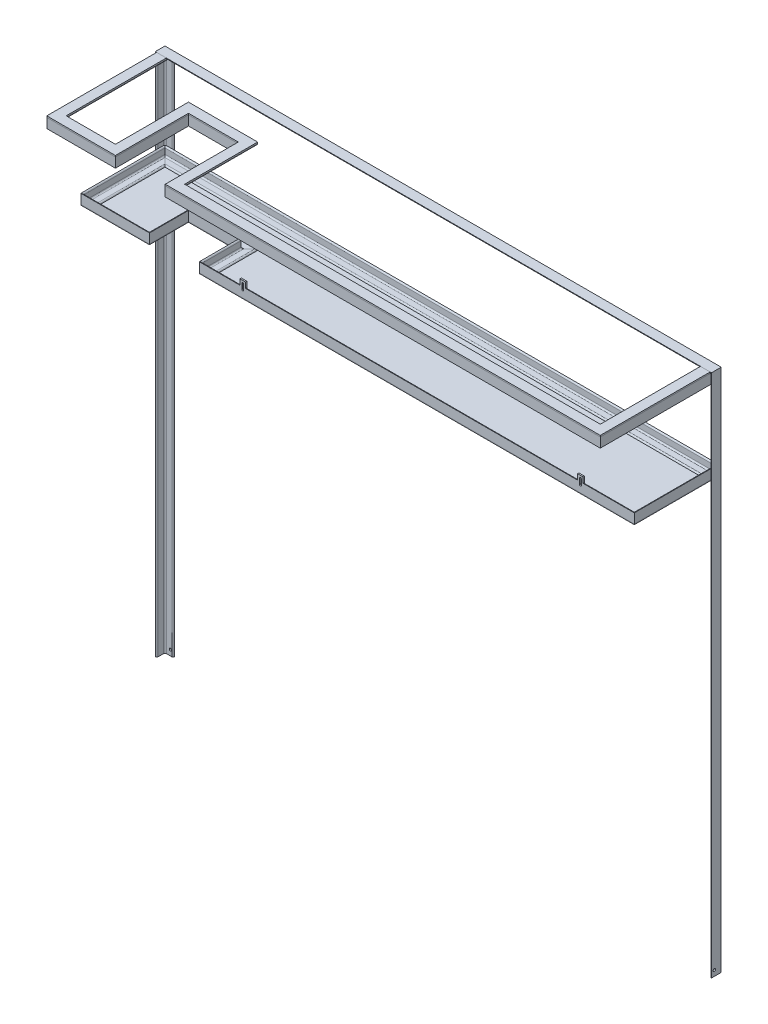
from build123d import *

# Parameters (mm, degrees)
MEMBER_1_DEPTH        = 1944.497474683
MEMBER_1_2_DEPTH      = 2060.497474683
MEMBER_1_2_DEPTH_BACK = 50.497474683
MEMBER_1_3_DEPTH      = 1944.497474683
MEMBER_2_DEPTH        = 477.497474683
MEMBER_2_2_DEPTH      = 348.994949366
MEMBER_2_3_DEPTH      = 364.994949366
MEMBER_2_4_DEPTH      = 280.994949366
MEMBER_2_5_DEPTH      = 364.994949366
MEMBER_2_6_DEPTH      = 1672.994949366
MEMBER_2_7_DEPTH      = 477.497474683
MEMBER_3_DEPTH        = 354.497474683
MEMBER_3_DEPTH_BACK   = 50.497474683
MEMBER_3_2_DEPTH      = 1672.994949366
MEMBER_3_3_DEPTH      = 241.994949366
MEMBER_3_4_DEPTH      = 280.994949366
MEMBER_3_5_DEPTH      = 241.994949366
MEMBER_3_6_DEPTH      = 348.994949366
MEMBER_3_7_DEPTH      = 404.994949366
MEMBER_3_8_DEPTH      = 2100.994949366
SKETCH_8_R            = 4.5
CUT_EXTRUDE_1_DEPTH   = 10
CUT_EXTRUDE_START     = -50
SKETCH_9_R            = 4.5
CUT_EXTRUDE_2_DEPTH   = 2440
EXTRUDE_1_DEPTH       = 5
EXTRUDE_2_DEPTH       = 2
SKETCH_14_W           = 20
SKETCH_14_H           = 30
EXTRUDE_3_DEPTH       = 5
CUT_EXTRUDE_3_DEPTH   = 5


with BuildPart() as part:
    # Sketch1 on segment 1 (carried to segment 1) → Member 1 (new body)
    with BuildSketch(Plane.ZX.offset(-1894)):
        with BuildLine():
            Line((0, 0), (0, 35))
            ThreePointArc((0, 35), (3.535533906, 33.535533906), (5, 30))
            Line((5, 30), (5, 10))
            ThreePointArc((5, 10), (6.464466094, 6.464466094), (10, 5))
            Line((10, 5), (30, 5))
            ThreePointArc((30, 5), (33.535533906, 3.535533906), (35, 0))
            Line((35, 0), (0, 0))
        make_face()
    extrude(amount=MEMBER_1_DEPTH)

    # Member 1 mitre 1
    split(bisect_by=Plane(origin=(0, 0, 0), x_dir=(0.707106781, -0.707106781, 0), z_dir=(-0.707106781, -0.707106781, 0)), keep=Keep.TOP)

    # 草图8 → 切除-拉伸1 (cut)
    with BuildSketch(Plane.XY.offset(5)):
        with Locations((25, -1874)):
            Circle(SKETCH_8_R)
        with Locations((2413, -1874)):
            Circle(SKETCH_8_R)
    extrude(amount=-CUT_EXTRUDE_1_DEPTH, mode=Mode.SUBTRACT)


with BuildPart() as body_2:
    # Sketch1 → Member 1 2 (new, two sides: drawn at the far end of the back side and taken through both)
    with BuildSketch(Plane(origin=(0, 0, 0), x_dir=(0, 0, 1), z_dir=(1, 0, 0)).offset(-MEMBER_1_2_DEPTH_BACK)):
        with BuildLine():
            Line((0, 0), (0, 35))
            ThreePointArc((0, 35), (3.535533906, 33.535533906), (5, 30))
            Line((5, 30), (5, 10))
            ThreePointArc((5, 10), (6.464466094, 6.464466094), (10, 5))
            Line((10, 5), (30, 5))
            ThreePointArc((30, 5), (33.535533906, 3.535533906), (35, 0))
            Line((35, 0), (0, 0))
        make_face()
    extrude(amount=MEMBER_1_2_DEPTH + MEMBER_1_2_DEPTH_BACK)

    # Member 1 2 mitre 1
    split(bisect_by=Plane(origin=(0, 0, 0), x_dir=(-0.707106781, 0.707106781, 0), z_dir=(0.707106781, 0.707106781, 0)), keep=Keep.TOP)

    # Member 1 2 mitre 2
    split(bisect_by=Plane(origin=(2010, 0, 0), x_dir=(-0.707106781, -0.707106781, 0), z_dir=(-0.707106781, 0.707106781, 0)), keep=Keep.TOP)


with BuildPart() as body_3:
    # Sketch1 on segment 3 (carried to segment 3) → Member 1 3 (new body)
    with BuildSketch(Plane(origin=(2010, 50.497474683, 0), x_dir=(0, 0, 1), z_dir=(0, -1, 0))):
        with BuildLine():
            Line((0, 0), (0, 35))
            ThreePointArc((0, 35), (3.535533906, 33.535533906), (5, 30))
            Line((5, 30), (5, 10))
            ThreePointArc((5, 10), (6.464466094, 6.464466094), (10, 5))
            Line((10, 5), (30, 5))
            ThreePointArc((30, 5), (33.535533906, 3.535533906), (35, 0))
            Line((35, 0), (0, 0))
        make_face()
    extrude(amount=MEMBER_1_3_DEPTH)

    # Member 1 3 mitre 1
    split(bisect_by=Plane(origin=(2010, 0, 0), x_dir=(0.707106781, 0.707106781, 0), z_dir=(0.707106781, -0.707106781, 0)), keep=Keep.TOP)

    # 草图9 → 切除-拉伸2 (cut)
    with BuildSketch(Plane.ZY.offset(CUT_EXTRUDE_START)):
        with Locations((25, -1874)):
            Circle(SKETCH_9_R)
    extrude(amount=-CUT_EXTRUDE_2_DEPTH, mode=Mode.SUBTRACT)


with BuildPart() as body_4:
    # Sketch11 → Member 2 (new body)
    with BuildSketch(Plane(origin=(5, -5, 5), x_dir=(0, -1, 0), z_dir=(0, 0, 1))):
        with BuildLine():
            Line((0, 0), (0, 35))
            ThreePointArc((0, 35), (3.535533906, 33.535533906), (5, 30))
            Line((5, 30), (5, 10))
            ThreePointArc((5, 10), (6.464466094, 6.464466094), (10, 5))
            Line((10, 5), (30, 5))
            ThreePointArc((30, 5), (33.535533906, 3.535533906), (35, 0))
            Line((35, 0), (0, 0))
        make_face()
    extrude(amount=MEMBER_2_DEPTH)

    # Member 2 mitre 1
    split(bisect_by=Plane(origin=(5, -5, 432), x_dir=(0, -1, 0), z_dir=(-0.707106781, 0, -0.707106781)), keep=Keep.TOP)


with BuildPart() as body_5:
    # Sketch11 on segment 2 (carried to segment 2) → Member 2 2 (new body)
    with BuildSketch(Plane(origin=(-45.497474683, -5, 432), x_dir=(0, -1, 0), z_dir=(1, 0, 0))):
        with BuildLine():
            Line((0, 0), (0, 35))
            ThreePointArc((0, 35), (3.535533906, 33.535533906), (5, 30))
            Line((5, 30), (5, 10))
            ThreePointArc((5, 10), (6.464466094, 6.464466094), (10, 5))
            Line((10, 5), (30, 5))
            ThreePointArc((30, 5), (33.535533906, 3.535533906), (35, 0))
            Line((35, 0), (0, 0))
        make_face()
    extrude(amount=MEMBER_2_2_DEPTH)

    # Member 2 2 mitre 1
    split(bisect_by=Plane(origin=(253, -5, 432), x_dir=(0, -1, 0), z_dir=(-0.707106781, 0, 0.707106781)), keep=Keep.TOP)

    # Member 2 2 mitre 2
    split(bisect_by=Plane(origin=(5, -5, 432), x_dir=(0, 1, 0), z_dir=(0.707106781, 0, 0.707106781)), keep=Keep.TOP)


with BuildPart() as body_6:
    # Sketch11 on segment 3 (carried to segment 3) → Member 2 3 (new body)
    with BuildSketch(Plane(origin=(253, -5, 482.497474683), x_dir=(0, -1, 0), z_dir=(0, 0, -1))):
        with BuildLine():
            Line((0, 0), (0, 35))
            ThreePointArc((0, 35), (3.535533906, 33.535533906), (5, 30))
            Line((5, 30), (5, 10))
            ThreePointArc((5, 10), (6.464466094, 6.464466094), (10, 5))
            Line((10, 5), (30, 5))
            ThreePointArc((30, 5), (33.535533906, 3.535533906), (35, 0))
            Line((35, 0), (0, 0))
        make_face()
    extrude(amount=MEMBER_2_3_DEPTH)

    # Member 2 3 mitre 1
    split(bisect_by=Plane(origin=(253, -5, 432), x_dir=(0, 1, 0), z_dir=(0.707106781, 0, -0.707106781)), keep=Keep.TOP)

    # Member 2 3 mitre 2
    split(bisect_by=Plane(origin=(253, -5, 168), x_dir=(0, -1, 0), z_dir=(-0.707106781, 0, 0.707106781)), keep=Keep.TOP)


with BuildPart() as body_7:
    # Sketch11 on segment 4 (carried to segment 4) → Member 2 4 (new body)
    with BuildSketch(Plane(origin=(202.502525317, -5, 168), x_dir=(0, -1, 0), z_dir=(1, 0, 0))):
        with BuildLine():
            Line((0, 0), (0, 35))
            ThreePointArc((0, 35), (3.535533906, 33.535533906), (5, 30))
            Line((5, 30), (5, 10))
            ThreePointArc((5, 10), (6.464466094, 6.464466094), (10, 5))
            Line((10, 5), (30, 5))
            ThreePointArc((30, 5), (33.535533906, 3.535533906), (35, 0))
            Line((35, 0), (0, 0))
        make_face()
    extrude(amount=MEMBER_2_4_DEPTH)

    # Member 2 4 mitre 1
    split(bisect_by=Plane(origin=(253, -5, 168), x_dir=(0, 1, 0), z_dir=(0.707106781, 0, -0.707106781)), keep=Keep.TOP)

    # Member 2 4 mitre 2
    split(bisect_by=Plane(origin=(433, -5, 168), x_dir=(0, -1, 0), z_dir=(-0.707106781, 0, -0.707106781)), keep=Keep.TOP)


with BuildPart() as body_8:
    # Sketch11 on segment 5 (carried to segment 5) → Member 2 5 (new body)
    with BuildSketch(Plane(origin=(433, -5, 117.502525317), x_dir=(0, -1, 0), z_dir=(0, 0, 1))):
        with BuildLine():
            Line((0, 0), (0, 35))
            ThreePointArc((0, 35), (3.535533906, 33.535533906), (5, 30))
            Line((5, 30), (5, 10))
            ThreePointArc((5, 10), (6.464466094, 6.464466094), (10, 5))
            Line((10, 5), (30, 5))
            ThreePointArc((30, 5), (33.535533906, 3.535533906), (35, 0))
            Line((35, 0), (0, 0))
        make_face()
    extrude(amount=MEMBER_2_5_DEPTH)

    # Member 2 5 mitre 1
    split(bisect_by=Plane(origin=(433, -5, 168), x_dir=(0, 1, 0), z_dir=(0.707106781, 0, 0.707106781)), keep=Keep.TOP)

    # Member 2 5 mitre 2
    split(bisect_by=Plane(origin=(433, -5, 432), x_dir=(0, -1, 0), z_dir=(-0.707106781, 0, -0.707106781)), keep=Keep.TOP)


with BuildPart() as body_9:
    # Sketch11 on segment 6 (carried to segment 6) → Member 2 6 (new body)
    with BuildSketch(Plane(origin=(382.502525317, -5, 432), x_dir=(0, -1, 0), z_dir=(1, 0, 0))):
        with BuildLine():
            Line((0, 0), (0, 35))
            ThreePointArc((0, 35), (3.535533906, 33.535533906), (5, 30))
            Line((5, 30), (5, 10))
            ThreePointArc((5, 10), (6.464466094, 6.464466094), (10, 5))
            Line((10, 5), (30, 5))
            ThreePointArc((30, 5), (33.535533906, 3.535533906), (35, 0))
            Line((35, 0), (0, 0))
        make_face()
    extrude(amount=MEMBER_2_6_DEPTH)

    # Member 2 6 mitre 1
    split(bisect_by=Plane(origin=(2005, -5, 432), x_dir=(0, -1, 0), z_dir=(-0.707106781, 0, 0.707106781)), keep=Keep.TOP)

    # Member 2 6 mitre 2
    split(bisect_by=Plane(origin=(433, -5, 432), x_dir=(0, 1, 0), z_dir=(0.707106781, 0, 0.707106781)), keep=Keep.TOP)


with BuildPart() as body_10:
    # Sketch11 on segment 7 (carried to segment 7) → Member 2 7 (new body)
    with BuildSketch(Plane(origin=(2005, -5, 482.497474683), x_dir=(0, -1, 0), z_dir=(0, 0, -1))):
        with BuildLine():
            Line((0, 0), (0, 35))
            ThreePointArc((0, 35), (3.535533906, 33.535533906), (5, 30))
            Line((5, 30), (5, 10))
            ThreePointArc((5, 10), (6.464466094, 6.464466094), (10, 5))
            Line((10, 5), (30, 5))
            ThreePointArc((30, 5), (33.535533906, 3.535533906), (35, 0))
            Line((35, 0), (0, 0))
        make_face()
    extrude(amount=MEMBER_2_7_DEPTH)

    # Member 2 7 mitre 1
    split(bisect_by=Plane(origin=(2005, -5, 432), x_dir=(0, 1, 0), z_dir=(0.707106781, 0, -0.707106781)), keep=Keep.TOP)


with BuildPart() as body_11:
    # Sketch12 → Member 3 (new, two sides: drawn at the far end of the back side and taken through both)
    with BuildSketch(Plane(origin=(2005, -339, 5), x_dir=(0, 1, 0), z_dir=(0, 0, 1)).offset(-MEMBER_3_DEPTH_BACK)):
        with BuildLine():
            Line((0, 0), (0, 35))
            ThreePointArc((0, 35), (3.535533906, 33.535533906), (5, 30))
            Line((5, 30), (5, 10))
            ThreePointArc((5, 10), (6.464466094, 6.464466094), (10, 5))
            Line((10, 5), (30, 5))
            ThreePointArc((30, 5), (33.535533906, 3.535533906), (35, 0))
            Line((35, 0), (0, 0))
        make_face()
    extrude(amount=MEMBER_3_DEPTH + MEMBER_3_DEPTH_BACK)

    # Member 3 mitre 1
    split(bisect_by=Plane(origin=(2005, -339, 5), x_dir=(0, 1, 0), z_dir=(0.707106781, 0, 0.707106781)), keep=Keep.TOP)

    # Member 3 mitre 2
    split(bisect_by=Plane(origin=(2005, -339, 309), x_dir=(0, 1, 0), z_dir=(0.707106781, 0, -0.707106781)), keep=Keep.TOP)


with BuildPart() as body_12:
    # Sketch12 on segment 2 (carried to segment 2) → Member 3 2 (new body)
    with BuildSketch(Plane(origin=(2055.497474683, -339, 309), x_dir=(0, 1, 0), z_dir=(-1, 0, 0))):
        with BuildLine():
            Line((0, 0), (0, 35))
            ThreePointArc((0, 35), (3.535533906, 33.535533906), (5, 30))
            Line((5, 30), (5, 10))
            ThreePointArc((5, 10), (6.464466094, 6.464466094), (10, 5))
            Line((10, 5), (30, 5))
            ThreePointArc((30, 5), (33.535533906, 3.535533906), (35, 0))
            Line((35, 0), (0, 0))
        make_face()
    extrude(amount=MEMBER_3_2_DEPTH)

    # Member 3 2 mitre 1
    split(bisect_by=Plane(origin=(2005, -339, 309), x_dir=(0, -1, 0), z_dir=(-0.707106781, 0, 0.707106781)), keep=Keep.TOP)

    # Member 3 2 mitre 2
    split(bisect_by=Plane(origin=(433, -339, 309), x_dir=(0, 1, 0), z_dir=(0.707106781, 0, 0.707106781)), keep=Keep.TOP)

    # 草图14 → 凸台-拉伸3 (add)
    with BuildSketch(Plane.XY.offset(309)):
        with Locations((590, -299)):
            Rectangle(SKETCH_14_W, SKETCH_14_H)
        with Locations((1810, -299)):
            Rectangle(SKETCH_14_W, SKETCH_14_H)
    extrude(amount=-EXTRUDE_3_DEPTH)

    # 草图15 → 切除-拉伸3 (cut)
    with BuildSketch(Plane(origin=(0, 0, 304), x_dir=(-1, 0, 0), z_dir=(0, 0, -1))):
        with BuildLine():
            Line((-1813.5, -294), (-1813.5, -314))
            ThreePointArc((-1813.5, -314), (-1810, -317.5), (-1806.5, -314))
            Line((-1806.5, -314), (-1806.5, -294))
            ThreePointArc((-1806.5, -294), (-1810, -290.5), (-1813.5, -294))
        make_face()
        with BuildLine():
            Line((-593.5, -294), (-593.5, -314))
            ThreePointArc((-593.5, -314), (-590, -317.5), (-586.5, -314))
            Line((-586.5, -314), (-586.5, -294))
            ThreePointArc((-586.5, -294), (-590, -290.5), (-593.5, -294))
        make_face()
    extrude(amount=-CUT_EXTRUDE_3_DEPTH, mode=Mode.SUBTRACT)


with BuildPart() as body_13:
    # Sketch12 on segment 3 (carried to segment 3) → Member 3 3 (new body)
    with BuildSketch(Plane(origin=(433, -339, 359.497474683), x_dir=(0, 1, 0), z_dir=(0, 0, -1))):
        with BuildLine():
            Line((0, 0), (0, 35))
            ThreePointArc((0, 35), (3.535533906, 33.535533906), (5, 30))
            Line((5, 30), (5, 10))
            ThreePointArc((5, 10), (6.464466094, 6.464466094), (10, 5))
            Line((10, 5), (30, 5))
            ThreePointArc((30, 5), (33.535533906, 3.535533906), (35, 0))
            Line((35, 0), (0, 0))
        make_face()
    extrude(amount=MEMBER_3_3_DEPTH)

    # Member 3 3 mitre 1
    split(bisect_by=Plane(origin=(433, -339, 309), x_dir=(0, -1, 0), z_dir=(-0.707106781, 0, -0.707106781)), keep=Keep.TOP)

    # Member 3 3 mitre 2
    split(bisect_by=Plane(origin=(433, -339, 168), x_dir=(0, 1, 0), z_dir=(0.707106781, 0, 0.707106781)), keep=Keep.TOP)


with BuildPart() as body_14:
    # Sketch12 on segment 4 (carried to segment 4) → Member 3 4 (new body)
    with BuildSketch(Plane(origin=(483.497474683, -339, 168), x_dir=(0, 1, 0), z_dir=(-1, 0, 0))):
        with BuildLine():
            Line((0, 0), (0, 35))
            ThreePointArc((0, 35), (3.535533906, 33.535533906), (5, 30))
            Line((5, 30), (5, 10))
            ThreePointArc((5, 10), (6.464466094, 6.464466094), (10, 5))
            Line((10, 5), (30, 5))
            ThreePointArc((30, 5), (33.535533906, 3.535533906), (35, 0))
            Line((35, 0), (0, 0))
        make_face()
    extrude(amount=MEMBER_3_4_DEPTH)

    # Member 3 4 mitre 1
    split(bisect_by=Plane(origin=(433, -339, 168), x_dir=(0, -1, 0), z_dir=(-0.707106781, 0, -0.707106781)), keep=Keep.TOP)

    # Member 3 4 mitre 2
    split(bisect_by=Plane(origin=(253, -339, 168), x_dir=(0, 1, 0), z_dir=(0.707106781, 0, -0.707106781)), keep=Keep.TOP)


with BuildPart() as body_15:
    # Sketch12 on segment 5 (carried to segment 5) → Member 3 5 (new body)
    with BuildSketch(Plane(origin=(253, -339, 117.502525317), x_dir=(0, 1, 0), z_dir=(0, 0, 1))):
        with BuildLine():
            Line((0, 0), (0, 35))
            ThreePointArc((0, 35), (3.535533906, 33.535533906), (5, 30))
            Line((5, 30), (5, 10))
            ThreePointArc((5, 10), (6.464466094, 6.464466094), (10, 5))
            Line((10, 5), (30, 5))
            ThreePointArc((30, 5), (33.535533906, 3.535533906), (35, 0))
            Line((35, 0), (0, 0))
        make_face()
    extrude(amount=MEMBER_3_5_DEPTH)

    # Member 3 5 mitre 1
    split(bisect_by=Plane(origin=(253, -339, 168), x_dir=(0, -1, 0), z_dir=(-0.707106781, 0, 0.707106781)), keep=Keep.TOP)

    # Member 3 5 mitre 2
    split(bisect_by=Plane(origin=(253, -339, 309), x_dir=(0, 1, 0), z_dir=(0.707106781, 0, -0.707106781)), keep=Keep.TOP)


with BuildPart() as body_16:
    # Sketch12 on segment 6 (carried to segment 6) → Member 3 6 (new body)
    with BuildSketch(Plane(origin=(303.497474683, -339, 309), x_dir=(0, 1, 0), z_dir=(-1, 0, 0))):
        with BuildLine():
            Line((0, 0), (0, 35))
            ThreePointArc((0, 35), (3.535533906, 33.535533906), (5, 30))
            Line((5, 30), (5, 10))
            ThreePointArc((5, 10), (6.464466094, 6.464466094), (10, 5))
            Line((10, 5), (30, 5))
            ThreePointArc((30, 5), (33.535533906, 3.535533906), (35, 0))
            Line((35, 0), (0, 0))
        make_face()
    extrude(amount=MEMBER_3_6_DEPTH)

    # Member 3 6 mitre 1
    split(bisect_by=Plane(origin=(253, -339, 309), x_dir=(0, -1, 0), z_dir=(-0.707106781, 0, 0.707106781)), keep=Keep.TOP)

    # Member 3 6 mitre 2
    split(bisect_by=Plane(origin=(5, -339, 309), x_dir=(0, 1, 0), z_dir=(0.707106781, 0, 0.707106781)), keep=Keep.TOP)


with BuildPart() as body_17:
    # Sketch12 on segment 7 (carried to segment 7) → Member 3 7 (new body)
    with BuildSketch(Plane(origin=(5, -339, 359.497474683), x_dir=(0, 1, 0), z_dir=(0, 0, -1))):
        with BuildLine():
            Line((0, 0), (0, 35))
            ThreePointArc((0, 35), (3.535533906, 33.535533906), (5, 30))
            Line((5, 30), (5, 10))
            ThreePointArc((5, 10), (6.464466094, 6.464466094), (10, 5))
            Line((10, 5), (30, 5))
            ThreePointArc((30, 5), (33.535533906, 3.535533906), (35, 0))
            Line((35, 0), (0, 0))
        make_face()
    extrude(amount=MEMBER_3_7_DEPTH)

    # Member 3 7 mitre 1
    split(bisect_by=Plane(origin=(5, -339, 309), x_dir=(0, -1, 0), z_dir=(-0.707106781, 0, -0.707106781)), keep=Keep.TOP)

    # Member 3 7 mitre 2
    split(bisect_by=Plane(origin=(5, -339, 5), x_dir=(0, -1, 0), z_dir=(-0.707106781, 0, 0.707106781)), keep=Keep.TOP)


with BuildPart() as body_18:
    # Sketch12 on segment 8 (carried to segment 8) → Member 3 8 (new body)
    with BuildSketch(Plane(origin=(-45.497474683, -339, 5), x_dir=(0, 1, 0), z_dir=(1, 0, 0))):
        with BuildLine():
            Line((0, 0), (0, 35))
            ThreePointArc((0, 35), (3.535533906, 33.535533906), (5, 30))
            Line((5, 30), (5, 10))
            ThreePointArc((5, 10), (6.464466094, 6.464466094), (10, 5))
            Line((10, 5), (30, 5))
            ThreePointArc((30, 5), (33.535533906, 3.535533906), (35, 0))
            Line((35, 0), (0, 0))
        make_face()
    extrude(amount=MEMBER_3_8_DEPTH)

    # Member 3 8 mitre 1
    split(bisect_by=Plane(origin=(2005, -339, 5), x_dir=(0, -1, 0), z_dir=(-0.707106781, 0, -0.707106781)), keep=Keep.TOP)

    # Member 3 8 mitre 2
    split(bisect_by=Plane(origin=(5, -339, 5), x_dir=(0, 1, 0), z_dir=(0.707106781, 0, -0.707106781)), keep=Keep.TOP)


with BuildPart() as body_19:
    # 草图11 → 凸台-拉伸1 (new body)
    with BuildSketch(Plane(origin=(0, -5, 0), x_dir=(1, 0, 0), z_dir=(0, 1, 0))):
        Polygon((2005, -35), (2005, -432), (433, -432), (433, -168), (253, -168), (253, -432), (5, -432), (5, -35), (40, -35), (40, -397), (218, -397), (218, -133), (468, -133), (468, -397), (1970, -397), (1970, -35), align=None)
    extrude(amount=EXTRUDE_1_DEPTH)


with BuildPart() as body_20:
    # 草图13 → 凸台-拉伸2 (new body)
    with BuildSketch(Plane.XZ.offset(339)):
        Polygon((5, 309), (5, 5), (2005, 5), (2005, 309), (433, 309), (433, 168), (253, 168), (253, 309), align=None)
    extrude(amount=EXTRUDE_2_DEPTH)


solid = Compound([part.part, body_2.part, body_3.part, body_4.part, body_5.part, body_6.part, body_7.part, body_8.part, body_9.part, body_10.part, body_11.part, body_12.part, body_13.part, body_14.part, body_15.part, body_16.part, body_17.part, body_18.part, body_19.part, body_20.part])
